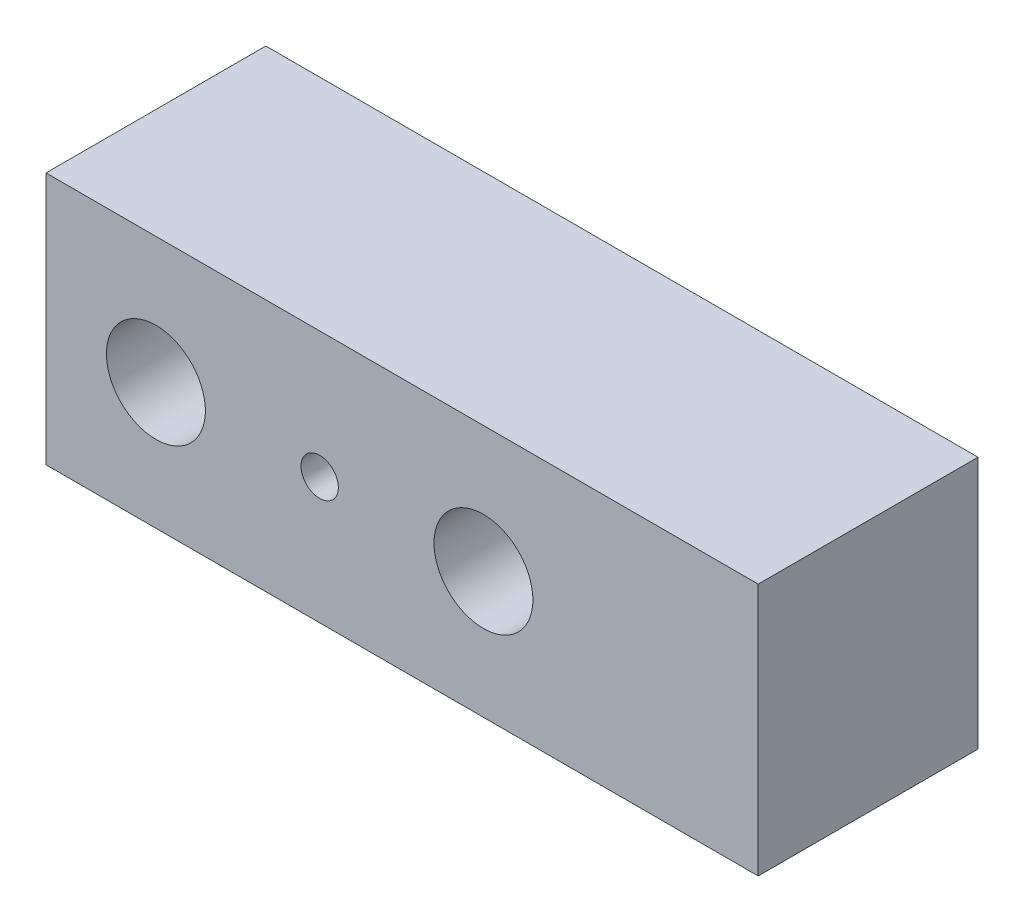
from build123d import *

# Parameters (mm, degrees)
SKETCH1_W                                           = 64.8
SKETCH1_H                                           = 20
BOSS_EXTRUDE1_DEPTH                                 = 23
SKETCH2_R                                           = 1.5
CUT_EXTRUDE1_DEPTH                                  = 20
CBORE_FOR_M8_HEX_SOCKET_HEAD_CAP_SCREW1_D           = 9
CBORE_FOR_M8_HEX_SOCKET_HEAD_CAP_SCREW1_DEPTH       = 41.94
CBORE_FOR_M8_HEX_SOCKET_HEAD_CAP_SCREW1_CBORE_D     = 15
CBORE_FOR_M8_HEX_SOCKET_HEAD_CAP_SCREW1_CBORE_DEPTH = 8.6
CBORE_FOR_M8_HEX_SOCKET_HEAD_CAP_SCREW1_TIP         = 2.703872786
CBORE_FOR_M3_HEX_SOCKET_HEAD_CAP_SCREW1_D           = 3.4
CBORE_FOR_M3_HEX_SOCKET_HEAD_CAP_SCREW1_DEPTH       = 41.94
CBORE_FOR_M3_HEX_SOCKET_HEAD_CAP_SCREW1_CBORE_D     = 6.5
CBORE_FOR_M3_HEX_SOCKET_HEAD_CAP_SCREW1_CBORE_DEPTH = 3.4
CBORE_FOR_M3_HEX_SOCKET_HEAD_CAP_SCREW1_TIP         = 1.021463052


with BuildPart() as part:
    # Sketch1 → Boss-Extrude1 (new body)
    with BuildSketch(Plane(origin=(0, 0, 0), x_dir=(1, 0, 0), z_dir=(0, 1, 0))):
        Rectangle(SKETCH1_W, SKETCH1_H)
    extrude(amount=BOSS_EXTRUDE1_DEPTH)

    # Sketch2 → Cut-Extrude1 (cut)
    with BuildSketch(Plane(origin=(0, 0, 0), x_dir=(1, 0, 0), z_dir=(0, 1, 0))):
        with Locations(Location((18.9, -6, 0), (0, 0, 270))):
            Circle(SKETCH2_R)
    extrude(amount=CUT_EXTRUDE1_DEPTH, mode=Mode.SUBTRACT)

    # CBORE for M8 Hex Socket Head Cap Screw1
    with Locations(Plane(origin=(-22.4, 11.5, -10), x_dir=(-1, 0, 0), z_dir=(0, 0, -1))):
        with Locations((0, 0), (-29.8, 0)):
            CounterBoreHole(CBORE_FOR_M8_HEX_SOCKET_HEAD_CAP_SCREW1_D / 2, CBORE_FOR_M8_HEX_SOCKET_HEAD_CAP_SCREW1_CBORE_D / 2, CBORE_FOR_M8_HEX_SOCKET_HEAD_CAP_SCREW1_CBORE_DEPTH, depth=CBORE_FOR_M8_HEX_SOCKET_HEAD_CAP_SCREW1_DEPTH)
            with Locations((0, 0, -(CBORE_FOR_M8_HEX_SOCKET_HEAD_CAP_SCREW1_DEPTH + CBORE_FOR_M8_HEX_SOCKET_HEAD_CAP_SCREW1_TIP / 2))):  # 118° drill point
                Cone(0, CBORE_FOR_M8_HEX_SOCKET_HEAD_CAP_SCREW1_D / 2, CBORE_FOR_M8_HEX_SOCKET_HEAD_CAP_SCREW1_TIP, mode=Mode.SUBTRACT)

    # CBORE for M3 Hex Socket Head Cap Screw1
    with Locations(Plane(origin=(-7.5, 11.5, -10), x_dir=(-1, 0, 0), z_dir=(0, 0, -1))):
        with Locations((0, 0)):
            CounterBoreHole(CBORE_FOR_M3_HEX_SOCKET_HEAD_CAP_SCREW1_D / 2, CBORE_FOR_M3_HEX_SOCKET_HEAD_CAP_SCREW1_CBORE_D / 2, CBORE_FOR_M3_HEX_SOCKET_HEAD_CAP_SCREW1_CBORE_DEPTH, depth=CBORE_FOR_M3_HEX_SOCKET_HEAD_CAP_SCREW1_DEPTH)
            with Locations((0, 0, -(CBORE_FOR_M3_HEX_SOCKET_HEAD_CAP_SCREW1_DEPTH + CBORE_FOR_M3_HEX_SOCKET_HEAD_CAP_SCREW1_TIP / 2))):  # 118° drill point
                Cone(0, CBORE_FOR_M3_HEX_SOCKET_HEAD_CAP_SCREW1_D / 2, CBORE_FOR_M3_HEX_SOCKET_HEAD_CAP_SCREW1_TIP, mode=Mode.SUBTRACT)


solid = part.part
